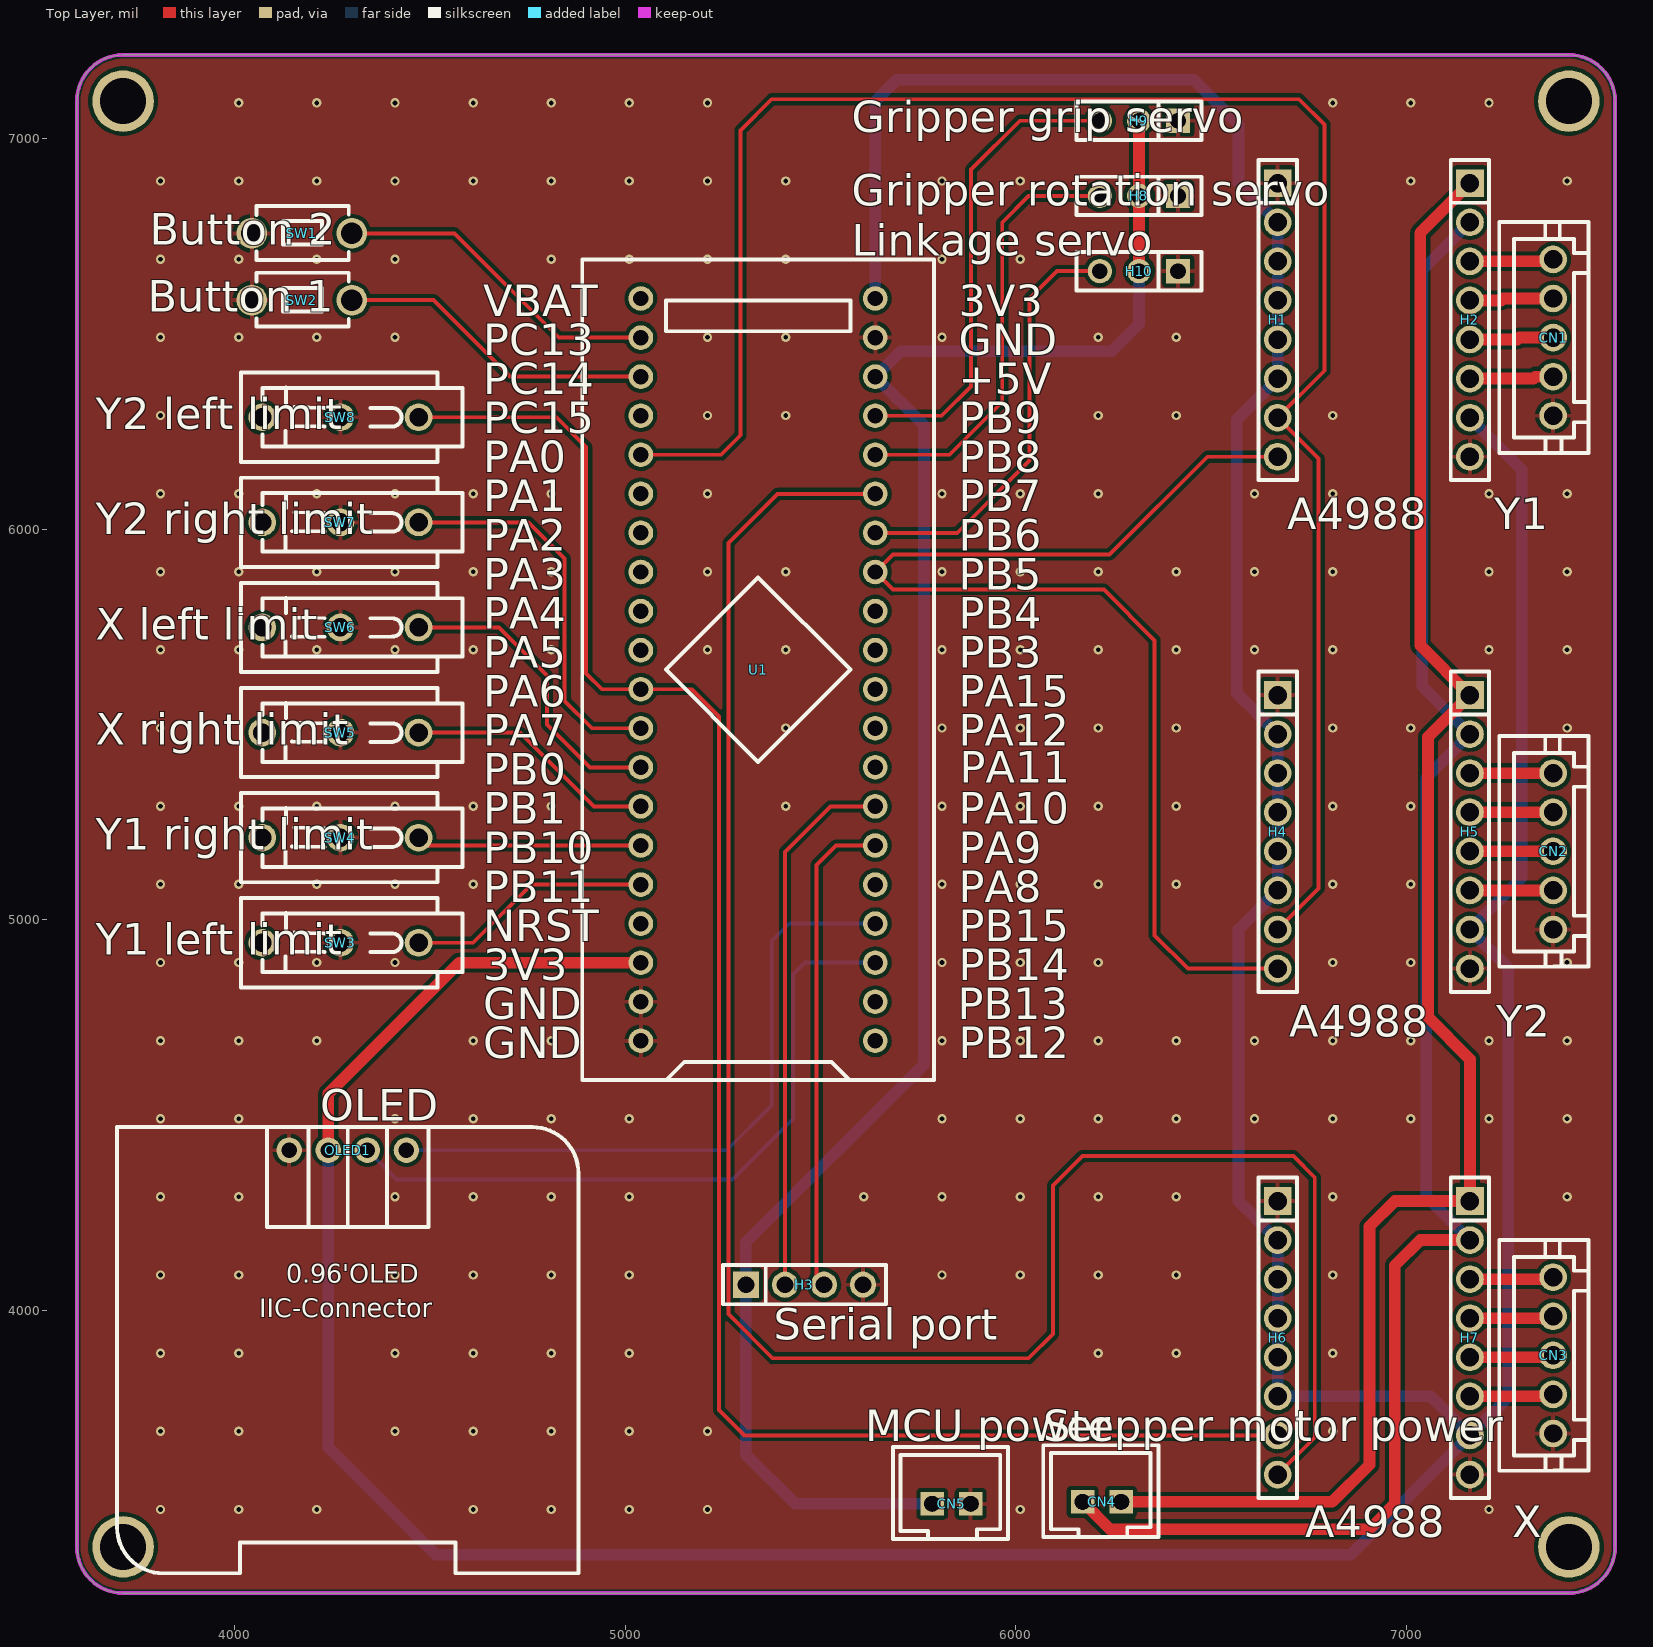
[diagram p0: Top Layer view]
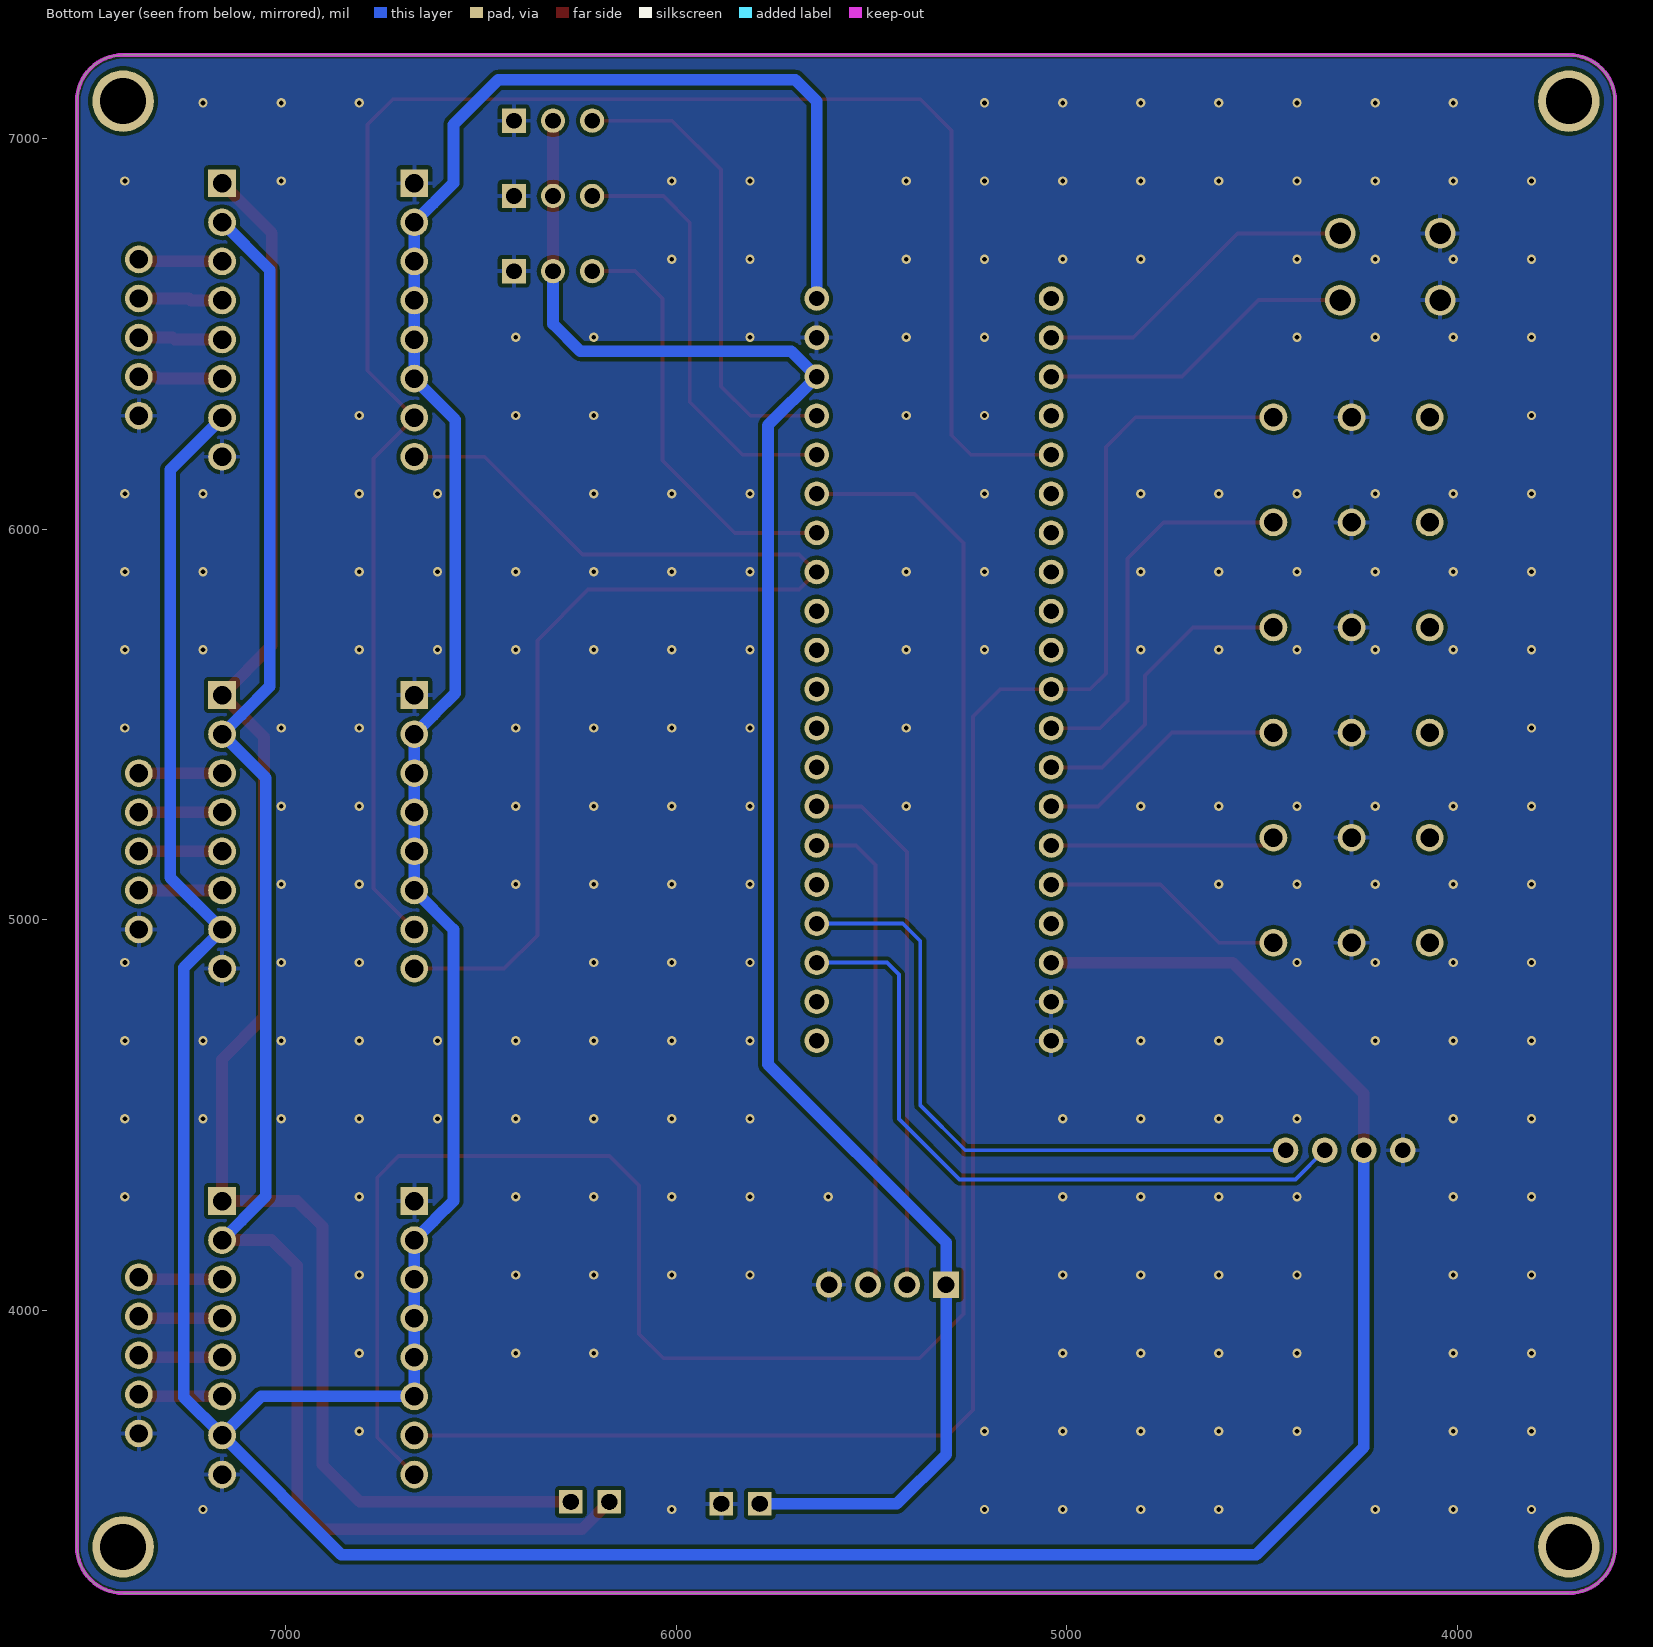
[diagram p1: Bottom Layer view, seen from below]
# Altium PCB MISC89043.pcbdoc
Units mil, origin at the board's own origin, x right, y up, seen from the top; angles counter-clockwise.
Board outline 3937.01 x 3937.01 mil, 2 copper layers (Top Layer, Bottom Layer), stack 62.206 mil thick; 25 components, 51 nets, 150 pads, 216 vias.

## Layer stack, top to bottom
Top Solder Mask Layer: solder mask 0.394, Dk 3.3
Top Layer: signal copper 1.379
Dielectric1: surface 59.449, FR4, Dk 4.5
Bottom Layer: signal copper 1.378
Bottom Solder Mask Layer: solder mask 0.394, Dk 3.3

## Board outline
3714.61,7213.5 ccw(c3714.61,7095.39) 3596.5,7095.39 3596.5,3394.61 ccw(c3714.61,3394.61) 3714.61,3276.5 7415.39,3276.5 ccw(c7415.39,3394.61) 7533.5,3394.61 7533.5,7095.39 ccw(c7415.39,7095.39) 7415.39,7213.5 3714.61,7213.5

## Design rules (kind name [scope] priority, off if disabled: settings)
BoardOutlineClearance copperThickness2oz_1 [All] p2 off: genericclearance=7.99 ignorepadtopadclearanceinfootprint=FALSE except(0: Arc-SplitContinuation Track-SplitContinuation SMDPad-SplitContinuation THPad-SplitContinuation Via-SplitContinuation Fill-SplitContinuation Region-SplitContinuation Poly-SplitContinuation Text-SplitContinuation Hole-SplitContinuation; 5.98: Arc-CutoutEdge Track-CutoutEdge SMDPad-CutoutEdge THPad-CutoutEdge Via-CutoutEdge Text-CutoutEdge; 6.9: Hole-OutlineEdge Hole-CutoutEdge; 10: Poly-OutlineEdge Poly-CutoutEdge; 11.81: Arc-OutlineEdge Track-OutlineEdge SMDPad-OutlineEdge THPad-OutlineEdge Via-OutlineEdge Fill-OutlineEdge Region-OutlineEdge Text-OutlineEdge Fill-CutoutEdge Region-CutoutEdge)
BoardOutlineClearance Plane_innerPlane_1 [All] p4 off: genericclearance=4.02 ignorepadtopadclearanceinfootprint=FALSE except(0: Arc-SplitContinuation Track-SplitContinuation SMDPad-SplitContinuation THPad-SplitContinuation Via-SplitContinuation Fill-SplitContinuation Region-SplitContinuation Poly-SplitContinuation Text-SplitContinuation Hole-SplitContinuation; 5.98: Arc-CutoutEdge Track-CutoutEdge SMDPad-CutoutEdge THPad-CutoutEdge Via-CutoutEdge Text-CutoutEdge; 6.9: Hole-OutlineEdge Hole-CutoutEdge; 10: Poly-OutlineEdge Poly-CutoutEdge; 11.81: Arc-OutlineEdge Track-OutlineEdge SMDPad-OutlineEdge THPad-OutlineEdge Via-OutlineEdge Fill-OutlineEdge Region-OutlineEdge Text-OutlineEdge Fill-CutoutEdge Region-CutoutEdge)
BoardOutlineClearance Copper_copperRegion_1 [All] p6 off: genericclearance=4.02 ignorepadtopadclearanceinfootprint=FALSE except(0: Arc-SplitContinuation Track-SplitContinuation SMDPad-SplitContinuation THPad-SplitContinuation Via-SplitContinuation Fill-SplitContinuation Region-SplitContinuation Poly-SplitContinuation Text-SplitContinuation Hole-SplitContinuation; 5.98: Arc-CutoutEdge Track-CutoutEdge SMDPad-CutoutEdge THPad-CutoutEdge Via-CutoutEdge Text-CutoutEdge; 6.9: Hole-OutlineEdge Hole-CutoutEdge; 10: Poly-OutlineEdge Poly-CutoutEdge; 11.81: Arc-OutlineEdge Track-OutlineEdge SMDPad-OutlineEdge THPad-OutlineEdge Via-OutlineEdge Fill-OutlineEdge Region-OutlineEdge Text-OutlineEdge Fill-CutoutEdge Region-CutoutEdge)
BoardOutlineClearance Copper_copperRegion_copperThickness1oz_1 [All] p8 off: genericclearance=4.02 ignorepadtopadclearanceinfootprint=FALSE except(0: Arc-SplitContinuation Track-SplitContinuation SMDPad-SplitContinuation THPad-SplitContinuation Via-SplitContinuation Fill-SplitContinuation Region-SplitContinuation Poly-SplitContinuation Text-SplitContinuation Hole-SplitContinuation; 5.98: Arc-CutoutEdge Track-CutoutEdge SMDPad-CutoutEdge THPad-CutoutEdge Via-CutoutEdge Text-CutoutEdge; 6.9: Hole-OutlineEdge Hole-CutoutEdge; 10: Poly-OutlineEdge Poly-CutoutEdge; 11.81: Arc-OutlineEdge Track-OutlineEdge SMDPad-OutlineEdge THPad-OutlineEdge Via-OutlineEdge Fill-OutlineEdge Region-OutlineEdge Text-OutlineEdge Fill-CutoutEdge Region-CutoutEdge)
BoardOutlineClearance Copper_copperRegion_Copper_copperRegion_1 [All] p10 off: genericclearance=4.02 ignorepadtopadclearanceinfootprint=FALSE except(0: Arc-SplitContinuation Track-SplitContinuation SMDPad-SplitContinuation THPad-SplitContinuation Via-SplitContinuation Fill-SplitContinuation Region-SplitContinuation Poly-SplitContinuation Text-SplitContinuation Hole-SplitContinuation; 5.98: Arc-CutoutEdge Track-CutoutEdge SMDPad-CutoutEdge THPad-CutoutEdge Via-CutoutEdge Text-CutoutEdge; 6.9: Hole-OutlineEdge Hole-CutoutEdge; 10: Poly-OutlineEdge Poly-CutoutEdge; 11.81: Arc-OutlineEdge Track-OutlineEdge SMDPad-OutlineEdge THPad-OutlineEdge Via-OutlineEdge Fill-OutlineEdge Region-OutlineEdge Text-OutlineEdge Fill-CutoutEdge Region-CutoutEdge)
BoardOutlineClearance copperThickness1oz_1 [All] p12: genericclearance=4.02 ignorepadtopadclearanceinfootprint=FALSE except(0: Arc-SplitContinuation Track-SplitContinuation SMDPad-SplitContinuation THPad-SplitContinuation Via-SplitContinuation Fill-SplitContinuation Region-SplitContinuation Poly-SplitContinuation Text-SplitContinuation Hole-SplitContinuation; 5.98: Arc-CutoutEdge Track-CutoutEdge SMDPad-CutoutEdge THPad-CutoutEdge Via-CutoutEdge Text-CutoutEdge; 6.9: Hole-OutlineEdge Hole-CutoutEdge; 10: Poly-OutlineEdge Poly-CutoutEdge; 11.81: Arc-OutlineEdge Track-OutlineEdge SMDPad-OutlineEdge THPad-OutlineEdge Via-OutlineEdge Fill-OutlineEdge Region-OutlineEdge Text-OutlineEdge Fill-CutoutEdge Region-CutoutEdge)
Clearance copperThickness2oz [All] p1 off: gap=7.99 ignorepadtopadclearanceinfootprint=FALSE except(5.98: SMDPad-Track SMDPad-SMDPad THPad-Track SMDPad-THPad THPad-THPad Track-Via SMDPad-Via THPad-Via Via-Via Fill-SMDPad Region-SMDPad Fill-THPad Region-THPad Fill-Via Region-Via Fill-Fill Fill-Region Region-Region Arc-Track Arc-SMDPad Arc-THPad Arc-Via Fill-Arc Region-Arc Arc-Arc Text-Track SMDPad-Text Text-THPad Text-Via Fill-Text Region-Text Arc-Text Text-Text; 6.9: Hole-Track Hole-SMDPad Hole-THPad Hole-Via Fill-Hole Region-Hole Hole-Arc Hole-Text; 10: Poly-Track Poly-SMDPad Poly-THPad Poly-Via Poly-Fill Poly-Region Poly-Poly Poly-Arc Poly-Text Poly-Hole; 11.81: Fill-Track Region-Track)
Clearance Plane_innerPlane [All] p3 off: gap=4.02 ignorepadtopadclearanceinfootprint=FALSE except(5.98: SMDPad-Track SMDPad-SMDPad THPad-Track SMDPad-THPad THPad-THPad Track-Via SMDPad-Via THPad-Via Via-Via Fill-SMDPad Region-SMDPad Fill-THPad Region-THPad Fill-Via Region-Via Fill-Fill Fill-Region Region-Region Arc-Track Arc-SMDPad Arc-THPad Arc-Via Fill-Arc Region-Arc Arc-Arc Text-Track SMDPad-Text Text-THPad Text-Via Fill-Text Region-Text Arc-Text Text-Text; 6.9: Hole-Track Hole-SMDPad Hole-THPad Hole-Via Fill-Hole Region-Hole Hole-Arc Hole-Text; 10: Poly-Track Poly-SMDPad Poly-THPad Poly-Via Poly-Fill Poly-Region Poly-Poly Poly-Arc Poly-Text Poly-Hole; 11.81: Fill-Track Region-Track)
Clearance Copper_copperRegion [All] p5 off: gap=4.02 ignorepadtopadclearanceinfootprint=FALSE except(5.98: SMDPad-Track SMDPad-SMDPad THPad-Track SMDPad-THPad THPad-THPad Track-Via SMDPad-Via THPad-Via Via-Via Fill-SMDPad Region-SMDPad Fill-THPad Region-THPad Fill-Via Region-Via Fill-Fill Fill-Region Region-Region Arc-Track Arc-SMDPad Arc-THPad Arc-Via Fill-Arc Region-Arc Arc-Arc Text-Track SMDPad-Text Text-THPad Text-Via Fill-Text Region-Text Arc-Text Text-Text; 6.9: Hole-Track Hole-SMDPad Hole-THPad Hole-Via Fill-Hole Region-Hole Hole-Arc Hole-Text; 10: Poly-Track Poly-SMDPad Poly-THPad Poly-Via Poly-Fill Poly-Region Poly-Poly Poly-Arc Poly-Text Poly-Hole; 11.81: Fill-Track Region-Track)
Clearance Copper_copperRegion_copperThickness1oz [All] p7 off: gap=4.02 ignorepadtopadclearanceinfootprint=FALSE except(5.98: SMDPad-Track SMDPad-SMDPad THPad-Track SMDPad-THPad THPad-THPad Track-Via SMDPad-Via THPad-Via Via-Via Fill-SMDPad Region-SMDPad Fill-THPad Region-THPad Fill-Via Region-Via Fill-Fill Fill-Region Region-Region Arc-Track Arc-SMDPad Arc-THPad Arc-Via Fill-Arc Region-Arc Arc-Arc Text-Track SMDPad-Text Text-THPad Text-Via Fill-Text Region-Text Arc-Text Text-Text; 6.9: Hole-Track Hole-SMDPad Hole-THPad Hole-Via Fill-Hole Region-Hole Hole-Arc Hole-Text; 10: Poly-Track Poly-SMDPad Poly-THPad Poly-Via Poly-Fill Poly-Region Poly-Poly Poly-Arc Poly-Text Poly-Hole; 11.81: Fill-Track Region-Track)
Clearance Copper_copperRegion_Copper_copperRegion [All] p9 off: gap=4.02 ignorepadtopadclearanceinfootprint=FALSE except(5.98: SMDPad-Track SMDPad-SMDPad THPad-Track SMDPad-THPad THPad-THPad Track-Via SMDPad-Via THPad-Via Via-Via Fill-SMDPad Region-SMDPad Fill-THPad Region-THPad Fill-Via Region-Via Fill-Fill Fill-Region Region-Region Arc-Track Arc-SMDPad Arc-THPad Arc-Via Fill-Arc Region-Arc Arc-Arc Text-Track SMDPad-Text Text-THPad Text-Via Fill-Text Region-Text Arc-Text Text-Text; 6.9: Hole-Track Hole-SMDPad Hole-THPad Hole-Via Fill-Hole Region-Hole Hole-Arc Hole-Text; 10: Poly-Track Poly-SMDPad Poly-THPad Poly-Via Poly-Fill Poly-Region Poly-Poly Poly-Arc Poly-Text Poly-Hole; 11.81: Fill-Track Region-Track)
Clearance copperThickness1oz [All] p11: gap=4.02 ignorepadtopadclearanceinfootprint=FALSE except(5.98: SMDPad-Track SMDPad-SMDPad THPad-Track SMDPad-THPad THPad-THPad Track-Via SMDPad-Via THPad-Via Via-Via Fill-SMDPad Region-SMDPad Fill-THPad Region-THPad Fill-Via Region-Via Fill-Fill Fill-Region Region-Region Arc-Track Arc-SMDPad Arc-THPad Arc-Via Fill-Arc Region-Arc Arc-Arc Text-Track SMDPad-Text Text-THPad Text-Via Fill-Text Region-Text Arc-Text Text-Text; 6.9: Hole-Track Hole-SMDPad Hole-THPad Hole-Via Fill-Hole Region-Hole Hole-Arc Hole-Text; 10: Poly-Track Poly-SMDPad Poly-THPad Poly-Via Poly-Fill Poly-Region Poly-Poly Poly-Arc Poly-Text Poly-Hole; 11.81: Fill-Track Region-Track)
DiffPairsRouting differentialPair [All] p1: maxlimit=6 minlimit=6 mostfreqgap=6 toplayer_minwidth=5 toplayer_prefwidth=10 toplayer_maxwidth=100 toplayer_mingap=6 toplayer_prefgap=6 toplayer_maxgap=6 bottomlayer_minwidth=5 bottomlayer_prefwidth=10 bottomlayer_maxwidth=100 bottomlayer_mingap=6 bottomlayer_prefgap=6 bottomlayer_maxgap=6 maxuncoupledlength=10
HoleToHoleClearance otherClearance [All] p1: gap=11.81 allowstackedmicrovias=TRUE
Length netLength [All] p1: minlimit=0 maxlimit=0
PasteMaskExpansion pasteMaskExpansion [All] p1: expansion=0
PlaneConnect innerPlane [All] p1: planeconnectstyle=Relief reliefexpansion=20 reliefentries=4 reliefconductorwidth=10 reliefairgap=10
PolygonConnect copperRegion_copperThickness1oz [All] p1 off: connectstyle=Relief reliefconductorwidth=10 reliefentries=4 polygonreliefangle="90 Angle" airgapwidth=10 via.connectstyle=Relief via.reliefconductorwidth=10 via.reliefentries=4 via.polygonreliefangle="90 Angle" via.airgapwidth=10
PolygonConnect copperRegion_Copper_copperRegion [All] p2 off: connectstyle=Relief reliefconductorwidth=10 reliefentries=4 polygonreliefangle="90 Angle" airgapwidth=10 via.connectstyle=Relief via.reliefconductorwidth=10 via.reliefentries=4 via.polygonreliefangle="90 Angle" via.airgapwidth=10
PolygonConnect copperRegion [All] p3: connectstyle=Relief reliefconductorwidth=10 reliefentries=4 polygonreliefangle="90 Angle" airgapwidth=10 via.connectstyle=Relief via.reliefconductorwidth=10 via.reliefentries=4 via.polygonreliefangle="90 Angle" via.airgapwidth=10
RoutingVias viaSize [All] p1: holewidth=12.01 width=24.02 viastyle="Through Hole" minholewidth=11.81 minwidth=19.68 maxholewidth=248.03 maxwidth=393.7
SolderMaskExpansion solderMaskExpansion [IsVia] p1: expansion=-1000 istentingtop=TRUE
SolderMaskExpansion solderMaskExpansion [All] p2: expansion=2 istentingtop=FALSE
Width copperThickness2oz_2 [All] p1 off: maxlimit=100 minlimit=8 preferedwidth=10
Width copperThickness1oz_2 [All] p2: maxlimit=100 minlimit=5 preferedwidth=10

## Components (designator, comment, footprint, x,y, rotation, side; value= is the part's Value field where it differs from the comment)
CN1 "XH2.54-5P" CONN-TH_5P-P2.54_C9900008095 7374.84,6490 r270 top
CN2 "XH2.54-5P" CONN-TH_5P-P2.54_C9900008095 7374.84,5175 r270 top
CN3 "XH2.54-5P" CONN-TH_5P-P2.54_C9900008095 7374.84,3885 r270 top
CN4 "XH2.54-2PIN-straight pin" CONN-TH_XH2.54-2P 6219.84,3510 r0 top
CN5 "XH2.54-2PIN-straight pin" CONN-TH_XH2.54-2P 5834.84,3505 r0 top
H1 "" HDR-TH_8P-P2.54-V-F-1 6669.84,6535 r270 top
H2 "" HDR-TH_8P-P2.54-V-F-1 7161.97,6535 r270 top
H3 "" HDR-TH_4P-P2.54-V-F 5458.7,4065.82 r0 top
H4 "" HDR-TH_8P-P2.54-V-F-1 6669.84,5225 r270 top
H5 "" HDR-TH_8P-P2.54-V-F-1 7161.97,5225 r270 top
H6 "" HDR-TH_8P-P2.54-V-F-1 6669.84,3930 r270 top
H7 "" HDR-TH_8P-P2.54-V-F-1 7161.97,3930 r270 top
H8 "" HDR-TH_3P-P2.54-V-F 6314.84,6852.5 r180 top
H9 "" HDR-TH_3P-P2.54-V-F 6314.84,7045 r180 top
H10 "" HDR-TH_3P-P2.54-V-F 6314.84,6660 r180 top
OLED1 "" 0.96OLED_4P 4289.84,4410 r0 top
SW1 "" Key_TH_3.5x6x4.3 4178.7,6756.82 r180 top
SW2 "" Key_TH_3.5x6x4.3 4178.7,6585.84 r180 top
SW3 "3JWD-DBHD-13.5 125" SW-TH_SHOU-HAN_3JWD-DBHD-13.5 4271,4941 r0 top
SW4 "3JWD-DBHD-13.5 125" SW-TH_SHOU-HAN_3JWD-DBHD-13.5 4271,5210 r0 top
SW5 "3JWD-DBHD-13.5 125" SW-TH_SHOU-HAN_3JWD-DBHD-13.5 4271,5479 r0 top
SW6 "3JWD-DBHD-13.5 125" SW-TH_SHOU-HAN_3JWD-DBHD-13.5 4271,5748 r0 top
SW7 "3JWD-DBHD-13.5 125" SW-TH_SHOU-HAN_3JWD-DBHD-13.5 4271,6017 r0 top
SW8 "3JWD-DBHD-13.5 125" SW-TH_SHOU-HAN_3JWD-DBHD-13.5 4271,6286 r0 top
U1 "STM32F103C8T6-Card" CONN-TH_L53.3-W22.9_STM32F103C8T6-CARD 5340,5640 r90 top

## Footprints (in the part's own frame and the unit in brackets; to place one, negate y for a bottom-side part, rotate by r counter-clockwise, add the part's x,y. Pads: shape width x height; smd on the part's side, far side on the other; paste and mask are expansions set on the pad)
0.96OLED_4P [mm]
  round 1.65 hole 1 copper offset 0,0: 1(-3.81,-0.001) 2(-1.27,0.002) 3(1.27,0.002) 4(3.81,0.002)
  silkscreen extent -15,-27.5 15,1.5
CONN-TH_5P-P2.54_C9900008095 [mm]
  round 1.8 hole 1.2 paste+0 mask+0.05: 1(-5.08,0) 2(-2.54,0) 3(0,0) 5(5.08,0)
  round 1.8 hole 1.2 copper offset 0,0 paste+0 mask+0.05: 4(2.54,0)
  silkscreen extent -7.5,-3.5 7.5,2.3
CONN-TH_L53.3-W22.9_STM32F103C8T6-CARD [mm]
  round 1.6 hole 1: 1(-24.13,-7.62) 2(-21.59,-7.62) 3(-19.05,-7.62) 4(-16.51,-7.62) 5(-13.97,-7.62) 6(-11.43,-7.62) 7(-8.89,-7.62) 8(-6.35,-7.62) 9(-3.81,-7.62) 10(-1.27,-7.62) 11(1.27,-7.62) 12(3.81,-7.62) 13(6.35,-7.62) 14(8.89,-7.62) 15(11.43,-7.62) 16(13.97,-7.62) 17(16.51,-7.62) 18(19.05,-7.62) 19(21.59,-7.62) 20(24.13,-7.62) 21(24.13,7.62) 22(21.59,7.62) 23(19.05,7.62) 24(16.51,7.62) 25(13.97,7.62) 26(11.43,7.62) 27(8.89,7.62) 28(6.35,7.62) 29(3.81,7.62) 30(1.27,7.62) 31(-1.27,7.62) 32(-3.81,7.62) 33(-6.35,7.62) 34(-8.89,7.62) 35(-11.43,7.62) 36(-13.97,7.62) 37(-16.51,7.62) 38(-19.05,7.62) 39(-21.59,7.62) 40(-24.13,7.62)
  silkscreen extent -26.67,-11.43 26.67,11.43
CONN-TH_XH2.54-2P [mil]
  rect 60x60 hole 39.37 slot 41.34 at 0 deg paste+0 mask+1.97: 1(-49.22,0) 2(49.21,0)
  silkscreen extent -150,-90 145,145
HDR-TH_3P-P2.54-V-F [mil]
  rect 62x62 hole 40.16: 1(-100,0)
  round 62 hole 40.16: 2(0,0) 3(100,0)
  silkscreen extent -160,-49 160,49
HDR-TH_4P-P2.54-V-F [mm]
  rect 1.7x1.7 hole 1.1: 1(-3.81,0)
  round 1.7 hole 1.1: 2(-1.27,0) 3(1.27,0) 4(3.81,0)
  silkscreen extent -5.29,-1.27 5.29,1.27
HDR-TH_8P-P2.54-V-F-1 [mm]
  rect 1.8x1.8 hole 1.2: 1(-8.89,0)
  round 1.8 hole 1.2: 2(-6.35,0) 3(-3.81,0) 4(-1.27,0) 5(1.27,0) 6(3.81,0) 7(6.35,0) 8(8.89,0)
  silkscreen extent -10.41,-1.25 10.41,1.25
Key_TH_3.5x6x4.3 [mil]
  round 78.7 hole 55.1 paste+0 mask+2: A(-121.44,0) B(134.46,0)
  silkscreen extent -114,-70 123,68
SW-TH_SHOU-HAN_3JWD-DBHD-13.5 [mm]
  round 1.8 hole 1.2: 1(-5.08,0) 2(0,0) 3(5.08,0)
  silkscreen extent -6.48,-2.9 7.92,2.9

## Free pads (board coordinates)
  round 157.48 hole 118.11: 1(3714.61,7095.39) 1(3714.61,3394.61) 1(7415.39,7095.39) 1(7415.39,3394.61)

## Via types
v1: diameter 24.02, hole 12, Top Layer to Bottom Layer, 216 vias

## Nets (pads, with @x,y where several pads share a name; then routed paths per layer and width w, separated by ;. In a path a pad name is that pad's centre, name@x,y a point inside that pad or via, vN(x,y) a via of type N, cw(c..) or ccw(c..) an arc to the next point about the centre after c; other vN are vias at no path point)
8-20V+: CN4.2 H2.1 H5.1 H7.1 | length 4368.2
  Top Layer w30: CN4.2 6809.84,3510 6904.84,3605 6904.84,4215 6969.84,4280 H7.1 7161.97,4642.87 7054.84,4750 7054.84,5467.87 H5.1 7034.84,5702.13 7034.84,6757.87 H2.1
8-20V-: CN4.1 H2.2 H5.2 H7.2 | length 4483.3
  Top Layer w30: CN4.1 6240.63,3440 6904.84,3440 6969.84,3505 6969.84,4115 7034.84,4180 H7.2
  Bottom Layer w30: H7.2 7114.79,4227.18 cw(c7126.54,4244.57) 7109.14,4232.82 7049.84,4292.13 7049.84,5362.87 H5.2 7114.79,5522.18 cw(c7126.54,5539.57) 7109.14,5527.82 7039.84,5597.13 7039.84,6662.87 H2.2
$1N17175: CN1.1 H2.3 | length 214.9
  Top Layer w30: H2.3 7369.84,6685 CN1.1@7374.84,6690
$1N17176: CN1.2 H2.4 | length 214.9
  Top Layer w30: H2.4 7241.57,6585 7246.57,6590 CN1.2@7374.84,6590
$1N17177: CN1.3 H2.5 | length 214.9
  Top Layer w30: H2.5 7282.99,6485 7287.99,6490 CN1.3@7374.84,6490
$1N17178: CN1.4 H2.6 | length 214.9
  Top Layer w30: H2.6 7324.42,6385 7329.41,6389.99 CN1.4@7374.84,6389.99
$1N17197: CN2.4 H5.6 | length 212.9
  Top Layer w30: H5.6 CN2.4@7374.83,5075
$1N17198: CN2.3 H5.5 | length 212.9
  Top Layer w30: H5.5 CN2.3@7374.84,5175
$1N17199: CN2.2 H5.4 | length 212.9
  Top Layer w30: H5.4 CN2.2@7374.84,5275
$1N17200: CN2.1 H5.3 | length 212.9
  Top Layer w30: H5.3 CN2.1@7374.84,5375
$1N17210: CN3.4 H7.6 | length 214.9
  Top Layer w30: H7.6 7369.85,3780 CN3.4@7374.84,3784.99
$1N17211: CN3.3 H7.5 | length 214.9
  Top Layer w30: H7.5 7369.84,3880 CN3.3@7374.84,3885
$1N17212: CN3.2 H7.4 | length 214.9
  Top Layer w30: H7.4 7369.84,3980 CN3.2@7374.84,3985
$1N17213: CN3.1 H7.3 | length 214.9
  Top Layer w30: H7.3 7369.84,4080 CN3.1@7374.84,4085
+5V: CN5.1 H3.1 H8.2 H9.2 H10.2 U1.18 | length 4779.4
  Top Layer w30: H10.2 H8.2 H9.2
  Bottom Layer w30: CN5.1 5434.84,3505 5308.7,3631.14 H3.1 5308.7,4173.86 5764.84,4630 5764.84,6265.16 U1.18 5705,6455 6244.84,6455 6314.84,6525 H10.2
GND: CN1.5 CN2.5 CN3.5 CN5.2 H1.1 H2.8 H3.4 H4.1 H5.8 H6.1 H7.8 H8.1 H9.1 H10.1 OLED1.1 SW1.B SW2.B SW3.2 SW4.2 SW5.2 SW6.2 SW7.2 SW8.2 U1.19 U1.39 U1.40
  other v1: 3810.6,3490.6 4010.6,3490.6 4210.6,3490.6 4610.6,3490.6 4810.6,3490.6 5010.6,3490.6 5210.6,3490.6 6010.6,3490.6 7210.6,3490.6 3810.6,3690.6 4010.6,3690.6 4410.6,3690.6 4610.6,3690.6 4810.6,3690.6 5010.6,3690.6 5210.6,3690.6 6810.6,3690.6 3810.6,3890.6 4010.6,3890.6 4410.6,3890.6 4610.6,3890.6 4810.6,3890.6 5010.6,3890.6 6210.6,3890.6 6410.6,3890.6 6810.6,3890.6 3810.6,4090.6 4010.6,4090.6 4410.6,4090.6 4610.6,4090.6 4810.6,4090.6 5010.6,4090.6 5810.6,4090.6 6010.6,4090.6 6210.6,4090.6 6410.6,4090.6 6810.6,4090.6 3810.6,4290.6 4010.6,4290.6 4410.6,4290.6 4610.6,4290.6 4810.6,4290.6 5010.6,4290.6 5610.6,4290.6 5810.6,4290.6 6010.6,4290.6 6210.6,4290.6 6410.6,4290.6 6810.6,4290.6 7410.6,4290.6 3810.6,4490.6 4010.6,4490.6 4410.6,4490.6 4610.6,4490.6 4810.6,4490.6 5010.6,4490.6 5810.6,4490.6 6010.6,4490.6 6210.6,4490.6 6410.6,4490.6 6610.6,4490.6 6810.6,4490.6 7010.6,4490.6 7210.6,4490.6 7410.6,4490.6 3810.6,4690.6 4010.6,4690.6 4210.6,4690.6 4610.6,4690.6 4810.6,4690.6 5810.6,4690.6 6010.6,4690.6 6210.6,4690.6 6410.6,4690.6 6610.6,4690.6 6810.6,4690.6 7010.6,4690.6 7210.6,4690.6 7410.6,4690.6 3810.6,4890.6 4010.6,4890.6 4210.6,4890.6 4410.6,4890.6 5810.6,4890.6 6010.6,4890.6 6210.6,4890.6 6810.6,4890.6 7010.6,4890.6 7410.6,4890.6 3810.6,5090.6 4010.6,5090.6 4210.6,5090.6 4410.6,5090.6 4610.6,5090.6 5810.6,5090.6 6010.6,5090.6 6210.6,5090.6 6410.6,5090.6 6810.6,5090.6 7010.6,5090.6 3810.6,5290.6 4010.6,5290.6 4210.6,5290.6 4410.6,5290.6 4610.6,5290.6 4810.6,5290.6 5410.6,5290.6 5810.6,5290.6 6010.6,5290.6 6210.6,5290.6 6410.6,5290.6 6810.6,5290.6 7010.6,5290.6 3810.6,5490.6 5410.6,5490.6 5810.6,5490.6 6010.6,5490.6 6210.6,5490.6 6410.6,5490.6 6810.6,5490.6 7010.6,5490.6 7410.6,5490.6 3810.6,5690.6 4010.6,5690.6 4210.6,5690.6 4410.6,5690.6 4610.6,5690.6 4810.6,5690.6 5210.6,5690.6 5410.6,5690.6 5810.6,5690.6 6010.6,5690.6 6210.6,5690.6 6410.6,5690.6 6610.6,5690.6 6810.6,5690.6 7210.6,5690.6 7410.6,5690.6 3810.6,5890.6 4010.6,5890.6 4210.6,5890.6 4410.6,5890.6 4610.6,5890.6 4810.6,5890.6 5210.6,5890.6 5410.6,5890.6 5810.6,5890.6 6010.6,5890.6 6210.6,5890.6 6410.6,5890.6 6610.6,5890.6 6810.6,5890.6 7210.6,5890.6 7410.6,5890.6 3810.6,6090.6 4010.6,6090.6 4210.6,6090.6 4410.6,6090.6 4610.6,6090.6 4810.6,6090.6 5210.6,6090.6 5810.6,6090.6 6010.6,6090.6 6210.6,6090.6 6610.6,6090.6 6810.6,6090.6 7210.6,6090.6 7410.6,6090.6 3810.6,6290.6 5210.6,6290.6 5410.6,6290.6 6210.6,6290.6 6410.6,6290.6 6810.6,6290.6 3810.6,6490.6 4010.6,6490.6 4210.6,6490.6 4410.6,6490.6 5210.6,6490.6 5410.6,6490.6 5810.6,6490.6 6210.6,6490.6 6410.6,6490.6 3810.6,6690.6 4010.6,6690.6 4210.6,6690.6 4410.6,6690.6 4810.6,6690.6 5010.6,6690.6 5210.6,6690.6 5410.6,6690.6 5810.6,6690.6 6010.6,6690.6 3810.6,6890.6 4010.6,6890.6 4210.6,6890.6 4410.6,6890.6 4610.6,6890.6 4810.6,6890.6 5010.6,6890.6 5210.6,6890.6 5410.6,6890.6 5810.6,6890.6 6010.6,6890.6 7010.6,6890.6 7410.6,6890.6 4010.6,7090.6 4210.6,7090.6 4410.6,7090.6 4610.6,7090.6 4810.6,7090.6 5010.6,7090.6 5210.6,7090.6 6810.6,7090.6 7010.6,7090.6 7210.6,7090.6
NRST: U1.37
PA0: H1.7 H4.7 U1.25 | length 4807.3
  Top Layer w10: U1.25 5244.85,6190 5294.84,6240 5294.84,7020 5374.84,7100 6724.84,7100 6789.84,7035 6789.84,6405 H1.7 6774.84,6180 6774.84,5080 H4.7
PA1: U1.26
PA2: U1.27
PA3: U1.28
PA4: U1.29
PA5: U1.30
PA6: H6.7 SW8.3 U1.31 | length 4657.8
  Top Layer w10: SW8.3 4823.85,6286 4899.84,6210 4899.84,5630 4939.84,5590 U1.31 5169.84,5590 5239.84,5520 5239.84,3745 5304.84,3680 H6.7
PA7: SW7.3 U1.32 | length 1001.1
  Top Layer w10: SW7.3 4752.85,6017 4844.84,5925 4844.84,5560 4914.84,5490 U1.32
PA8: U1.5
PA9: H3.3 U1.6 | length 1252.9
  Top Layer w10: H3.3 5489.84,4084.68 5489.84,5140 5539.85,5190 U1.6
PA10: H3.2 U1.7 | length 1387.4
  Top Layer w10: H3.2 5408.7,5173.86 5524.85,5290 U1.7
PA11: U1.8
PA12: U1.9
PA15: U1.10
PB0: SW6.3 U1.33 | length 790.5
  Top Layer w10: SW6.3 4676.85,5748 4799.84,5625 4799.84,5500 4909.84,5390 U1.33
PB1: SW5.3 U1.34 | length 647.3
  Top Layer w10: SW5.3 4730.85,5479 4919.84,5290 U1.34
PB3: U1.11
PB4: U1.12
PB5: H1.8 H4.8 U1.13 | length 3044.6
  Top Layer w10: H4.8 6439.84,4875 6354.84,4960 6354.84,5715 6224.84,5845 5685,5845 U1.13 5685,5935 6239.84,5935 6489.84,6185 H1.8
PB6: H10.3 U1.14 | length 1095.5
  Top Layer w10: U1.14 5849.85,5990 6034.84,6175 6034.84,6590 6104.84,6660 H10.3
PB7: H6.8 U1.15 | length 5208.1
  Top Layer w10: U1.15 5389.85,6090 5264.25,5964.41 5264.25,3990.59 5377.34,3877.5 6032.34,3877.5 6094.84,3940 6094.84,4320 6169.84,4395 6709.84,4395 6764.84,4340 6764.84,3675 H6.8
PB8: H8.3 U1.16 | length 1118.7
  Top Layer w10: U1.16 5829.85,6190 5964.84,6325 5964.84,6785 6032.34,6852.5 H8.3
PB9: H9.3 U1.17 | length 1212.7
  Top Layer w10: U1.17 5809.85,6290 5884.84,6365 5884.84,6920 6009.84,7045 H9.3
PB10: SW4.3 U1.35 | length 577.3
  Top Layer w10: SW4.3 4490.99,5190 U1.35
PB11: SW3.3 U1.36 | length 630.7
  Top Layer w10: SW3.3 4610.84,4941 4759.85,5090 U1.36
PB12: U1.1
PB13: U1.2
PB14: OLED1.3 U1.3 | length 1777.9
  Bottom Layer w10: OLED1.3@4339.84,4410.05 4414.89,4335 5274.84,4335 5429.84,4490 5429.84,4860 5459.85,4890 U1.3
PB15: OLED1.4 U1.4 | length 1686.4
  Bottom Layer w10: OLED1.4@4439.84,4410.05 5259.89,4410.05 5374.84,4525 5374.84,4945 5419.85,4990 U1.4
PC13: SW1.A U1.22 | length 850.4
  Top Layer w10: SW1.A 4563.02,6756.82 4829.84,6490 U1.22
PC14: SW2.A U1.23 | length 821
  Top Layer w10: SW2.A 4509,6585.84 4704.84,6390 U1.23
PC15: U1.24
VBAT: U1.21
VCC: H1.2 H1.3 H1.4 H1.5 H1.6 H2.7 H4.2 H4.3 H4.4 H4.5 H4.6 H5.7 H6.2 H6.3 H6.4 H6.5 H6.6 H7.7 OLED1.2 U1.20 U1.38 | length 13307.7
  Top Layer w30: OLED1.2@4239.84,4410.05 4239.84,4555 4574.85,4890 U1.38
  Bottom Layer w30: OLED1.2@4239.84,4410.05 4239.84,3650 4514.84,3375 6856.97,3375 H7.7 ; U1.20 5640,7095.16 5694.84,7150 6454.84,7150 6569.84,7035 6569.84,6885 6617.02,6837.82 ccw(c6634.41,6849.57) 6622.67,6832.18 H1.2 H1.3 H1.4 H1.5 H1.6 6564.84,6280 6564.84,5580 6617.02,5527.82 ccw(c6634.41,5539.57) 6622.67,5522.18 H4.2 H4.3 H4.4 H4.5 H4.6 6569.84,4975 6569.84,4280 6617.02,4232.82 ccw(c6634.41,4244.57) 6622.67,4227.18 H6.2 H6.3 H6.4 H6.5 H6.6 7061.97,3780 H7.7 ; H2.7 7294.84,6152.13 7294.84,5107.87 H5.7 7259.84,4877.13 7259.84,3777.87 H7.7
pads on no net: SW3.1 SW4.1 SW5.1 SW6.1 SW7.1 SW8.1

## Polygon pours and split planes (outlines as drawn)
GND on Bottom Layer (solid, remove dead copper, pour order 4): 3525,7335 3525,3170 7700,3170 7700,7335
GND on Top Layer (solid, remove dead copper, pour order 2): 3000,7505 3000,3090 7930,3090 7930,7505
GND on Top Layer (solid, remove dead copper, pour order 4): 3479.84,7550 3479.84,3000 7824.84,3000 7824.84,7550

## Keep-outs
Board Outline Layer:
  the board outline again, w10

## Silkscreen, mask and mechanical layers (free items; w line width, h text height)
Top Silkscreen Layer:
  text "Gripper grip servo" at 5580.08,7015 h80
  text "Gripper rotation servo" at 5580.08,6827.93 h80
  text "Button 2" at 3783.03,6727.68 h80
  text "Linkage servo" at 5579.84,6700 h80
  text "Button 1" at 3777.92,6555.94 h80
  text "VBAT" at 4635.95,6545 h80
  text "3V3" at 5854.16,6545 h80
  text "PC13" at 4635.95,6445 h80
  text "GND" at 5854.16,6445 h80
  text "PC14" at 4635.95,6345 h80
  text "+5V" at 5854.16,6345 h80
  text "Y2 left limit" at 3644.84,6255 h80
  text "PC15" at 4635.95,6245 h80
  text "PB9" at 5854.16,6245 h80
  text "PA0" at 4635.95,6145 h80
  text "PB8" at 5854.16,6145 h80
  text "PA1" at 4635.95,6045 h80
  text "PB7" at 5854.16,6045 h80
  text "A4988     Y1" at 6694.84,6000 h80
  text "Y2 right limit" at 3644.84,5986 h80
  text "PA2" at 4635.95,5945 h80
  text "PB6" at 5854.16,5945 h80
  text "PA3" at 4635.95,5845 h80
  text "PB5" at 5854.16,5845 h80
  text "PA4" at 4635.95,5745 h80
  text "PB4" at 5854.16,5745 h80
  text "X left limit" at 3644.84,5717 h80
  text "PA5" at 4635.95,5645 h80
  text "PB3" at 5854.16,5645 h80
  text "PA6" at 4635.95,5545 h80
  text "PA15" at 5854.16,5545 h80
  text "X right limit" at 3644.84,5448 h80
  text "PA7" at 4635.95,5445 h80
  text "PA12" at 5854.16,5445 h80
  text "PA11" at 5855.95,5350 h80
  text "PB0" at 4635.95,5345 h80
  text "PB1" at 4635.95,5245 h80
  text "PA10" at 5854.16,5245 h80
  text "Y1 right limit" at 3644.84,5179 h80
  text "PB10" at 4635.95,5145 h80
  text "PA9" at 5854.16,5145 h80
  text "PB11" at 4635.95,5045 h80
  text "PA8" at 5854.16,5045 h80
  text "NRST" at 4635.95,4945 h80
  text "PB15" at 5854.16,4945 h80
  text "Y1 left limit" at 3644.84,4910 h80
  text "3V3" at 4635.95,4845 h80
  text "PB14" at 5854.16,4845 h80
  text "GND" at 4635.95,4745 h80
  text "PB13" at 5850.95,4745 h80
  text "A4988     Y2" at 6699.84,4700 h80
  text "GND" at 4635.95,4645 h80
  text "PB12" at 5854.16,4645 h80
  text "OLED" at 4219.84,4485 h80
  text "Serial port" at 5379.84,3925 h80
  text "MCU power" at 5614.84,3665 h80
  text "Stepper motor power" at 6069.84,3665 h80
  text "A4988     X" at 6739.84,3420 h80